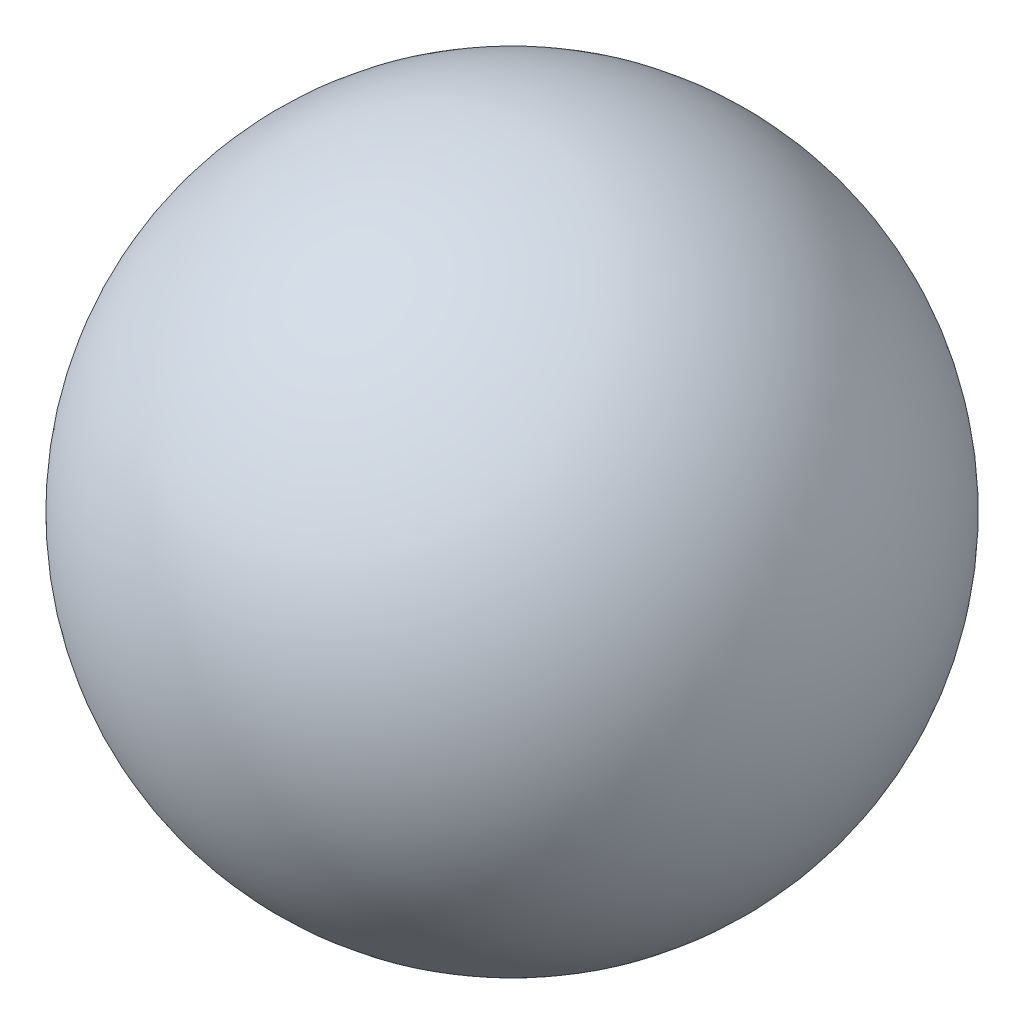
SolidWorks part; units mm, degrees
material "GCr15"
ref_plane "Front Plane" through (0, 0, 0) normal (0, 0, 1) x (1, 0, 0)
ref_plane "Top Plane" through (0, 0, 0) normal (0, 1, 0) x (1, 0, 0)
ref_plane "Right Plane" through (0, 0, 0) normal (1, 0, 0) x (0, 0, -1)
sketch "Sketch1" plane through (0, 0, 0) normal (0, 0, 1) x (1, 0, 0)
  line L0 (0, 1.65) -> (0, -1.65)
  arc A0 (0, -1.65) -> (0, 1.65) centre (0, 0) ccw
  dimension "D1" = 3.3
revolve "Revolve1" add sketch "Sketch1" angle 360 about L0
